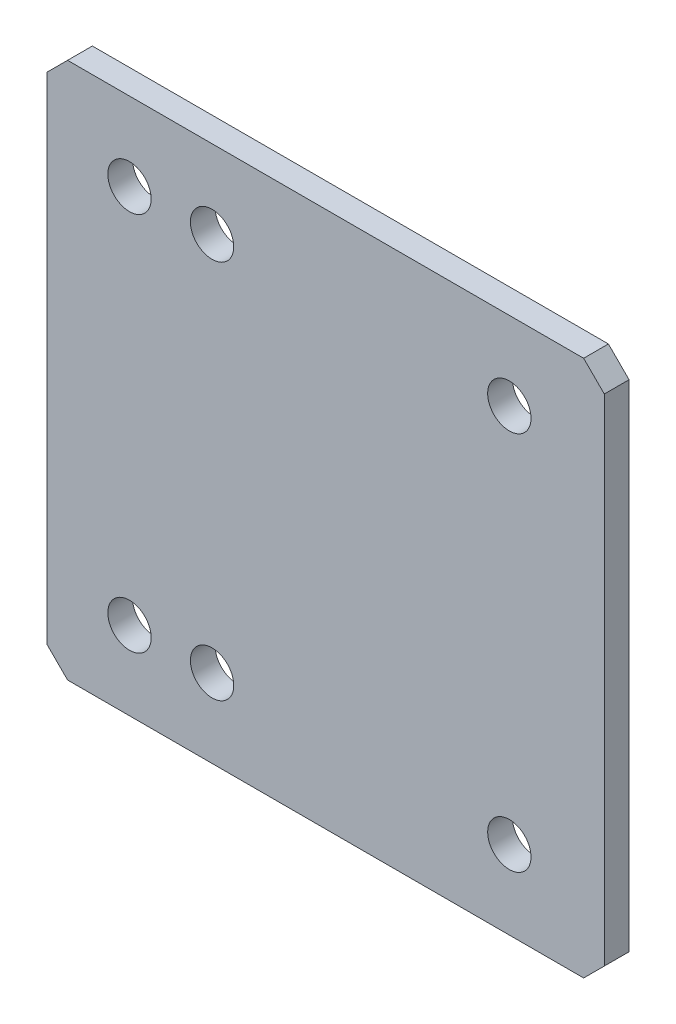
from build123d import *

# Parameters (mm, degrees)
SKETCH1_R           = 5.25
BOSS_EXTRUDE1_DEPTH = 3


with BuildPart() as part:
    # Sketch1 → Boss-Extrude1 (new, symmetric)
    with BuildSketch(Plane.XY):
        Polygon((-67.5, 60), (-62.5, 65), (62.5, 65), (67.5, 60), (67.5, -60), (62.5, -65), (-62.5, -65), (-67.5, -60), align=None)
        with Locations((-47.5, 46)):
            Circle(SKETCH1_R, mode=Mode.SUBTRACT)
        with Locations((-27.5, 46)):
            Circle(SKETCH1_R, mode=Mode.SUBTRACT)
        with Locations((44.5, 46)):
            Circle(SKETCH1_R, mode=Mode.SUBTRACT)
        with Locations(Location((44.5, -46, 0), (0, 0, 180))):
            Circle(SKETCH1_R, mode=Mode.SUBTRACT)
        with Locations(Location((-27.5, -46, 0), (0, 0, 180))):
            Circle(SKETCH1_R, mode=Mode.SUBTRACT)
        with Locations(Location((-47.5, -46, 0), (0, 0, 180))):
            Circle(SKETCH1_R, mode=Mode.SUBTRACT)
    extrude(amount=BOSS_EXTRUDE1_DEPTH, both=True)


solid = part.part
